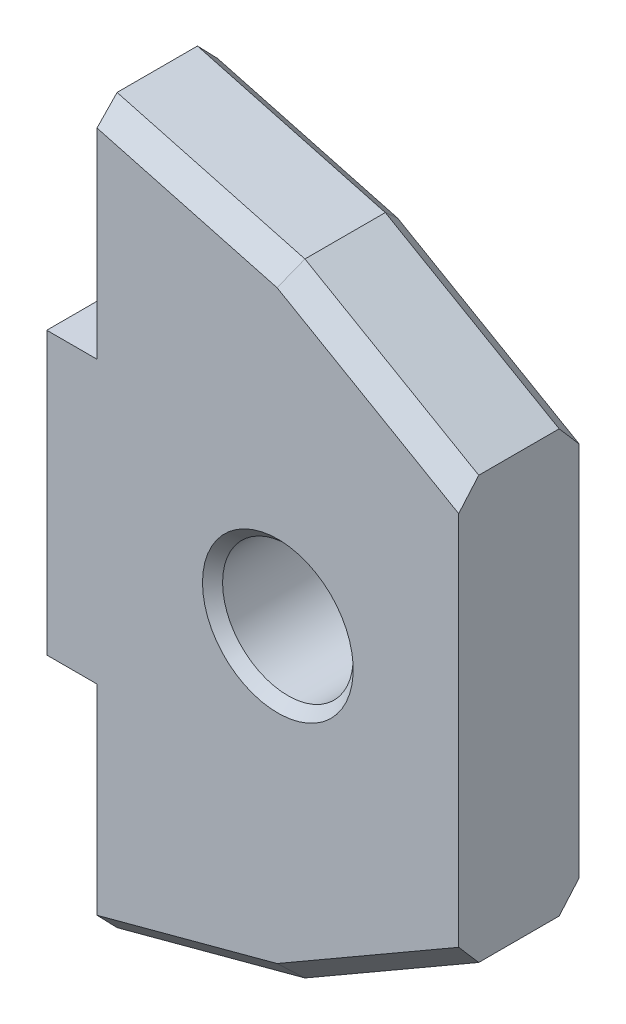
from build123d import *

# Parameters (mm, degrees)
SKETCH1_R           = 6.5
BOSS_EXTRUDE1_DEPTH = 6
CHAMFER1_SIZE       = 2
CHAMFER2_SIZE       = 1


with BuildPart() as part:
    # Sketch1 → Boss-Extrude1 (new, symmetric)
    with BuildSketch(Plane.XY):
        Polygon((-23, -14), (-23, 14), (-18, 14), (-18, 36), (0.696152423, 30.990381057), (18, 21), (18, -21), (0.696152423, -30.990381057), (-18, -36), (-18, -14), align=None)
        with Locations(Location((0, 0, 0), (0, 0, 180))):
            Circle(SKETCH1_R, mode=Mode.SUBTRACT)
    extrude(amount=BOSS_EXTRUDE1_DEPTH, both=True)

    # Chamfer1
    chamfer1_edges = [part.edges().sort_by_distance(p)[0] for p in [
        (-8.651923789, -33.495190528, -6),
        (9.348076211, -25.995190528, -6),
        (9.348076211, 25.995190528, 6),
        (9.348076211, 25.995190528, -6),
        (-8.651923789, 33.495190528, -6),
        (9.348076211, -25.995190528, 6),
        (-8.651923789, -33.495190528, 6),
        (-8.651923789, 33.495190528, 6),
    ]]
    chamfer(chamfer1_edges, length=CHAMFER1_SIZE)

    # Chamfer2
    chamfer2_edges = [part.edges().sort_by_distance(p)[0] for p in [
        (6.5, 0, 6),
        (6.5, 0, -6),
    ]]
    chamfer(chamfer2_edges, length=CHAMFER2_SIZE)


solid = part.part
